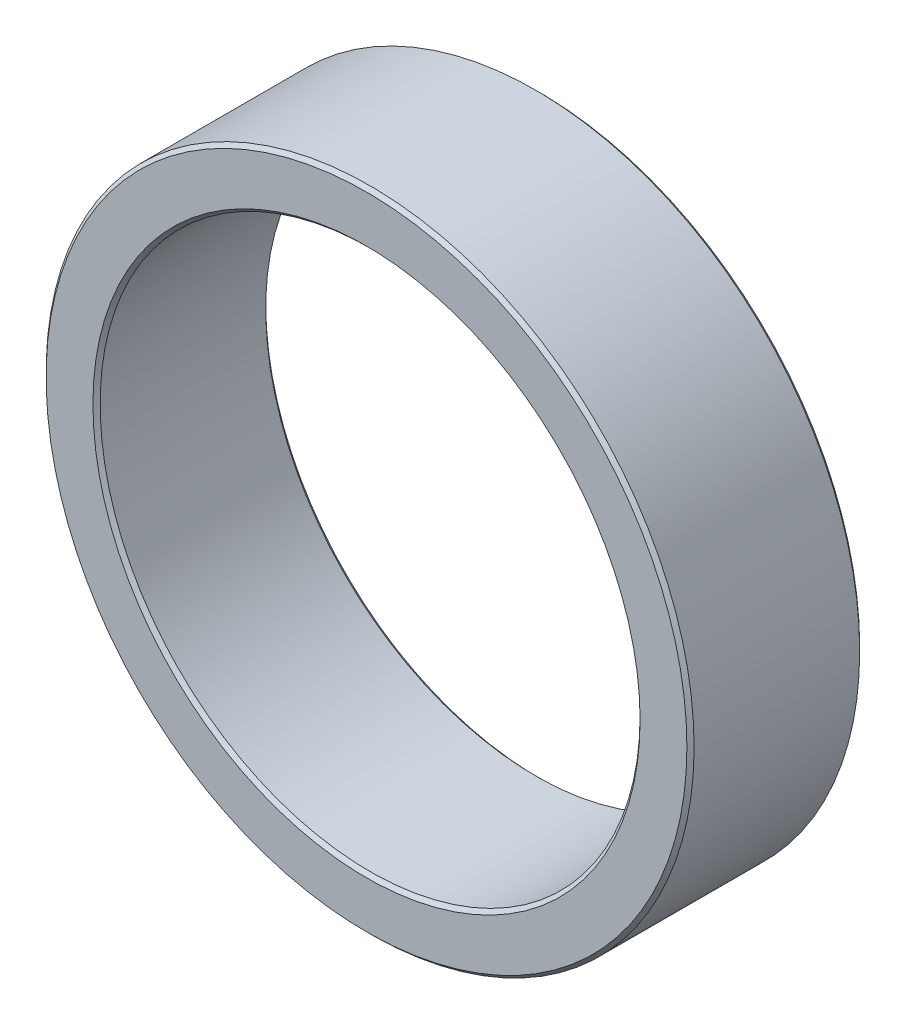
SolidWorks part; units mm, degrees
ref_plane "Front Plane" through (0, 0, 0) normal (0, 0, 1) x (1, 0, 0)
ref_plane "Top Plane" through (0, 0, 0) normal (0, 1, 0) x (1, 0, 0)
ref_plane "Right Plane" through (0, 0, 0) normal (1, 0, 0) x (0, 0, -1)
sketch "Sketch1" plane through (0, 0, 0) normal (0, 0, 1) x (1, 0, 0)
  circle A0 centre (0, 0) radius 45
  circle A1 centre (0, 0) radius 37.5
  dimension "D1" = 75
  dimension "D2" = 90
extrude "Boss-Extrude1" add sketch "Sketch1" along normal blind 24
chamfer "Chamfer1" distance 0.5 angle 45 4 edges at (37.5, 0, 0) (45, 0, 0) (37.5, 0, 24) (45, 0, 24)
